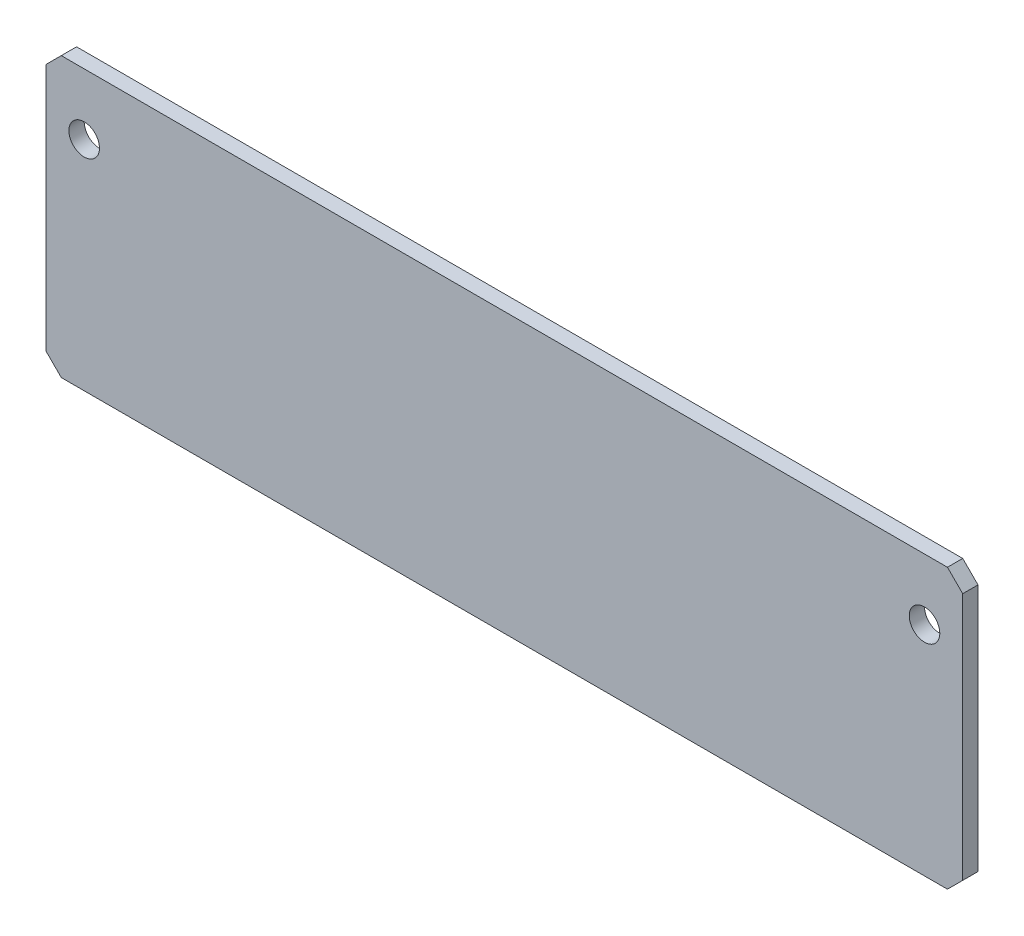
SolidWorks part; units mm, degrees
ref_plane "Front Plane" through (0, 0, 0) normal (0, 0, 1) x (1, 0, 0)
ref_plane "Top Plane" through (0, 0, 0) normal (0, 1, 0) x (1, 0, 0)
ref_plane "Right Plane" through (0, 0, 0) normal (1, 0, 0) x (0, 0, -1)
sketch "Sketch1" plane through (0, 0, 0) normal (0, 0, 1) x (1, 0, 0)
  line L1 (-600, 182.5) -> (600, 182.5)
  line L2 (-600, 182.5) -> (-600, -182.5)
  line L3 (-600, -182.5) -> (600, -182.5)
  line L4 (600, 182.5) -> (600, -182.5)
  line L5 (-600, 182.5) -> (600, -182.5) construction
  line L6 (-600, -182.5) -> (600, 182.5) construction
  point P0 (0, 0)
  dimension "D1" = 1200
  dimension "D2" = 365
extrude "Boss-Extrude1" add sketch "Sketch1" along normal blind 20
sketch "Sketch2" plane through (0, 0, 20) normal (0, 0, 1) x (1, 0, 0)
  line L0 (-600, 182.5) -> (-600, -182.5) construction
  line L1 (600, 182.5) -> (-600, 182.5) construction
  line L2 (0, 386.4853) -> (0, -409.0258) construction
  circle A0 centre (-550, 102.5) radius 20
  circle A1 centre (550, 102.5) radius 20
  dimension "D3" = 40
  dimension "D1" = 50
  dimension "D2" = 80
extrude "Cut-Extrude1" cut sketch "Sketch2" against normal through all both and the other way through all
chamfer "Chamfer1" distance 20 angle 45 2 edges at (600, 182.5, 10) (-600, 182.5, 10)
chamfer "Chamfer2" distance 20 angle 45 2 edges at (-600, -182.5, 10) (600, -182.5, 10)
